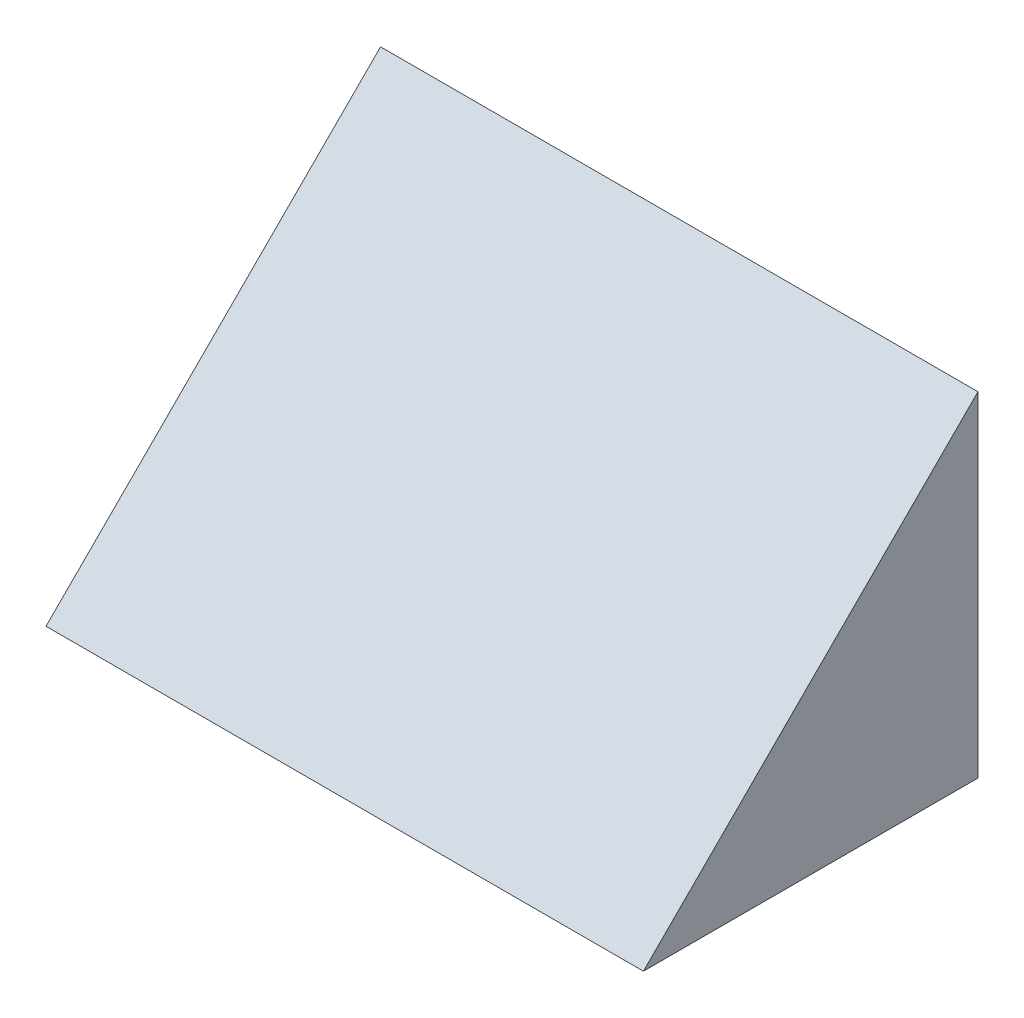
from build123d import *

# Parameters (mm, degrees)
SKETCH1_W               = 80
SKETCH1_H               = 400
BOSS_EXTRUDE1_DEPTH     = 80
BOSS_EXTRUDE2_DEPTH     = 80
CUT_EXTRUDE1_DEPTH      = 300
BOSS_EXTRUDE3_DEPTH     = 500
CUT_EXTRUDE2_DEPTH      = 718.63500472
CUT_EXTRUDE2_DEPTH_BACK = 718.63500472


with BuildPart() as part:
    # Sketch1 → Boss-Extrude1 (new body)
    with BuildSketch(Plane.XY):
        Rectangle(SKETCH1_W, SKETCH1_H)
    extrude(amount=BOSS_EXTRUDE1_DEPTH)

    # Sketch2 → Boss-Extrude2 (add)
    with BuildSketch(Plane.ZY.offset(40)):
        Polygon((0, -200), (400, -200), (0, 200), align=None)
    extrude(amount=-BOSS_EXTRUDE2_DEPTH)

    # Sketch3 → Cut-Extrude1 (cut)
    with BuildSketch(Plane.ZY.offset(40)):
        Polygon((80, 120), (0, 200), (172.987961084, 200), align=None)
    extrude(amount=-CUT_EXTRUDE1_DEPTH, mode=Mode.SUBTRACT)

    # Sketch4 → Boss-Extrude3 (add)
    with BuildSketch(Plane.ZY.offset(40)):
        Polygon((0, -200), (0, 250), (450, -200), align=None)
    extrude(amount=-BOSS_EXTRUDE3_DEPTH)

    # Sketch5 → Cut-Extrude2 (cut, two sides: drawn at the far end of the back side and taken through both)
    with BuildSketch(Plane.ZY.offset(40).offset(-CUT_EXTRUDE2_DEPTH_BACK)):
        Polygon((280, -200), (0, 80), (0, 250), (450, -200), align=None)
    extrude(amount=CUT_EXTRUDE2_DEPTH + CUT_EXTRUDE2_DEPTH_BACK, mode=Mode.SUBTRACT)


solid = part.part
